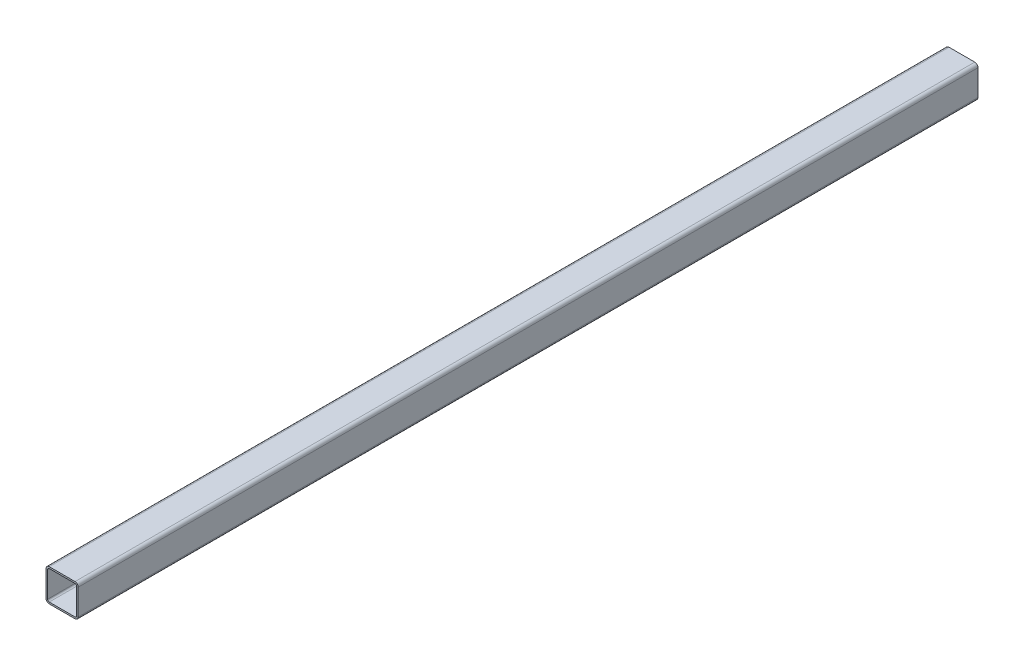
SolidWorks part; units mm, degrees
material "Q235A"
ref_plane "Front Plane" through (0, 0, 0) normal (0, 0, 1) x (1, 0, 0)
ref_plane "Top Plane" through (0, 0, 0) normal (0, 1, 0) x (1, 0, 0)
ref_plane "Right Plane" through (0, 0, 0) normal (1, 0, 0) x (0, 0, -1)
sketch "Sketch1" plane through (0, 0, 0) normal (0, 0, 1) x (1, 0, 0)
  line L1 (-20, 20) -> (20, 20)
  line L2 (-20, 20) -> (-20, -20)
  line L3 (-20, -20) -> (20, -20)
  line L4 (20, 20) -> (20, -20)
  line L5 (-20, 20) -> (20, -20) construction
  line L6 (-20, -20) -> (20, 20) construction
  line L7 (-18, 18) -> (18, 18)
  line L8 (-18, 18) -> (-18, -18)
  line L9 (-18, -18) -> (18, -18)
  line L10 (18, 18) -> (18, -18)
  line L11 (-18, 18) -> (18, -18) construction
  line L12 (-18, -18) -> (18, 18) construction
  point P0 (0, 0)
  point P6 (0, 0)
  dimension "D1" = 40
  dimension "D2" = 40
  dimension "D3" = 2
  dimension "D4" = 2
extrude "Boss-Extrude1" add sketch "Sketch1" along normal blind 1116
fillet "Fillet1" radius 2 4 edges at (18, 18, 558) (-18, 18, 558) (-18, -18, 558) (18, -18, 558)
fillet "Fillet2" radius 4 4 edges at (20, 20, 558) (20, -20, 558) (-20, 20, 558) (-20, -20, 558)
